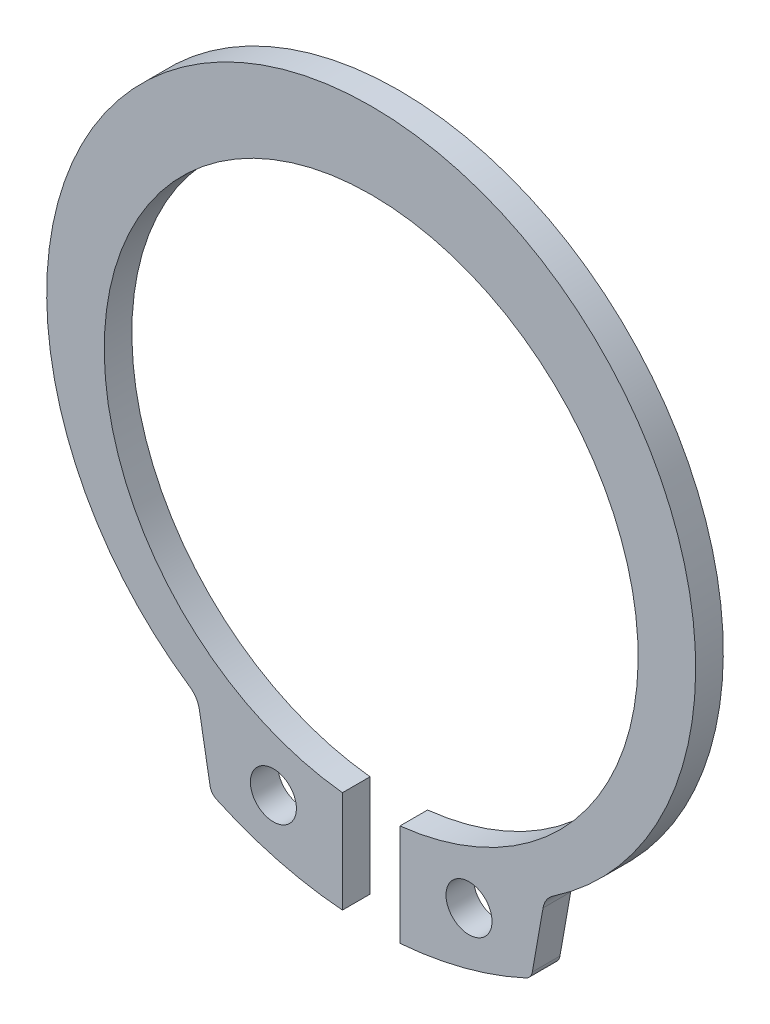
from build123d import *

# Parameters (mm, degrees)
SKETCH_1_R      = 1
EXTRUDE_1_DEPTH = 1.2


with BuildPart() as part:
    # 草图1 → 凸台-拉伸1 (new body)
    with BuildSketch(Plane(origin=(0, 0, -1.2), x_dir=(-1, 0, 0), z_dir=(0, 0, -1))):
        with BuildLine():
            Line((-1.25, -16.781097141), (-1.25, -12.362454205))
            ThreePointArc((-1.25, -12.362454205), (0, 10.77), (1.25, -12.362454205))
            Line((1.25, -12.362454205), (1.25, -16.781097141))
            ThreePointArc((1.25, -16.781097141), (4.048302979, -16.309381221), (6.719258119, -15.350728987))
            ThreePointArc((6.719258119, -15.350728987), (6.905510397, -15.201919327), (7.00168518, -14.983780295))
            Line((7.00168518, -14.983780295), (7.468086116, -12.338689143))
            ThreePointArc((7.468086116, -12.338689143), (7.614025765, -11.968002587), (7.893099573, -11.68370571))
            ThreePointArc((7.893099573, -11.68370571), (0, 14.1), (-7.893099573, -11.68370571))
            ThreePointArc((-7.893099573, -11.68370571), (-7.614025765, -11.968002587), (-7.468086116, -12.338689143))
            Line((-7.468086116, -12.338689143), (-7.00168518, -14.983780295))
            ThreePointArc((-7.00168518, -14.983780295), (-6.905510397, -15.201919327), (-6.719258119, -15.350728987))
            ThreePointArc((-6.719258119, -15.350728987), (-4.048302979, -16.309381221), (-1.25, -16.781097141))
        make_face()
        with Locations(Location((-4.25, -13.959261213, 0), (0, 0, 180))):
            Circle(SKETCH_1_R, mode=Mode.SUBTRACT)
        with Locations(Location((4.25, -13.959261213, 0), (0, 0, 180))):
            Circle(SKETCH_1_R, mode=Mode.SUBTRACT)
    extrude(amount=-EXTRUDE_1_DEPTH)


solid = part.part
